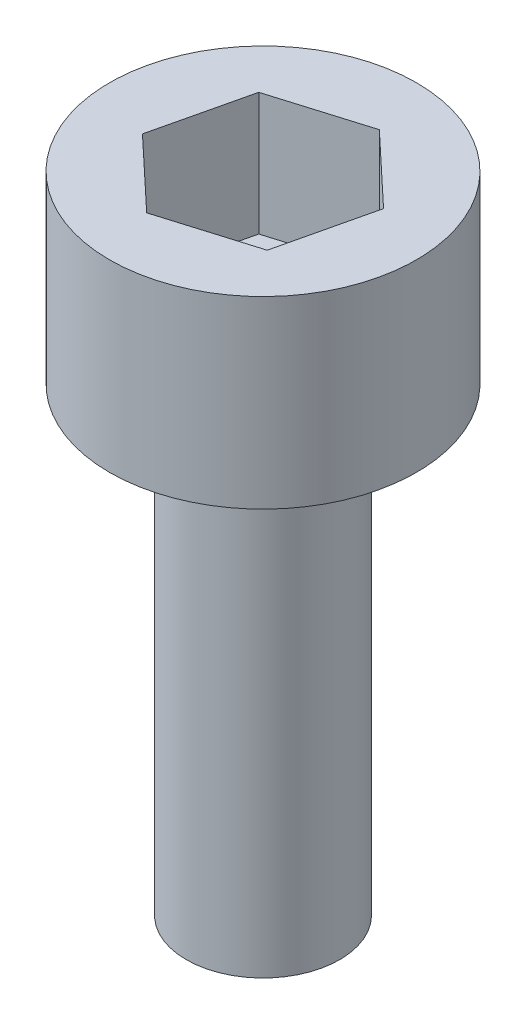
SolidWorks part; units mm, degrees
ref_plane "Front Plane" through (0, 0, 0) normal (0, 0, 1) x (1, 0, 0)
ref_plane "Top Plane" through (0, 0, 0) normal (0, 1, 0) x (1, 0, 0)
ref_plane "Right Plane" through (0, 0, 0) normal (1, 0, 0) x (0, 0, -1)
sketch "Sketch1" plane through (0, 0, 0) normal (0, 1, 0) x (1, 0, 0)
  circle A0 centre (0, 0) radius 5
  dimension "D1" = 10
extrude "Boss-Extrude1" add sketch "Sketch1" along normal blind 30
sketch "Sketch2" plane through (0, 30, 0) normal (0, 1, 0) x (1, 0, 0)
  circle A0 centre (0, 0) radius 10
  dimension "D1" = 20
extrude "Boss-Extrude2" add sketch "Sketch2" along normal blind 12
sketch "Sketch3" plane through (0, 42, 0) normal (0, 1, 0) x (1, 0, 0)
  line L1 (4.5939, -4.3186) -> (6.0369, 1.8192)
  line L2 (6.0369, 1.8192) -> (1.443, 6.1377)
  line L3 (1.443, 6.1377) -> (-4.5939, 4.3186)
  line L4 (-4.5939, 4.3186) -> (-6.0369, -1.8192)
  line L5 (-6.0369, -1.8192) -> (-1.443, -6.1377)
  line L6 (-1.443, -6.1377) -> (4.5939, -4.3186)
  circle A0 centre (0, 0) radius 5.4603 construction
extrude "Cut-Extrude1" cut sketch "Sketch3" against normal blind 8
